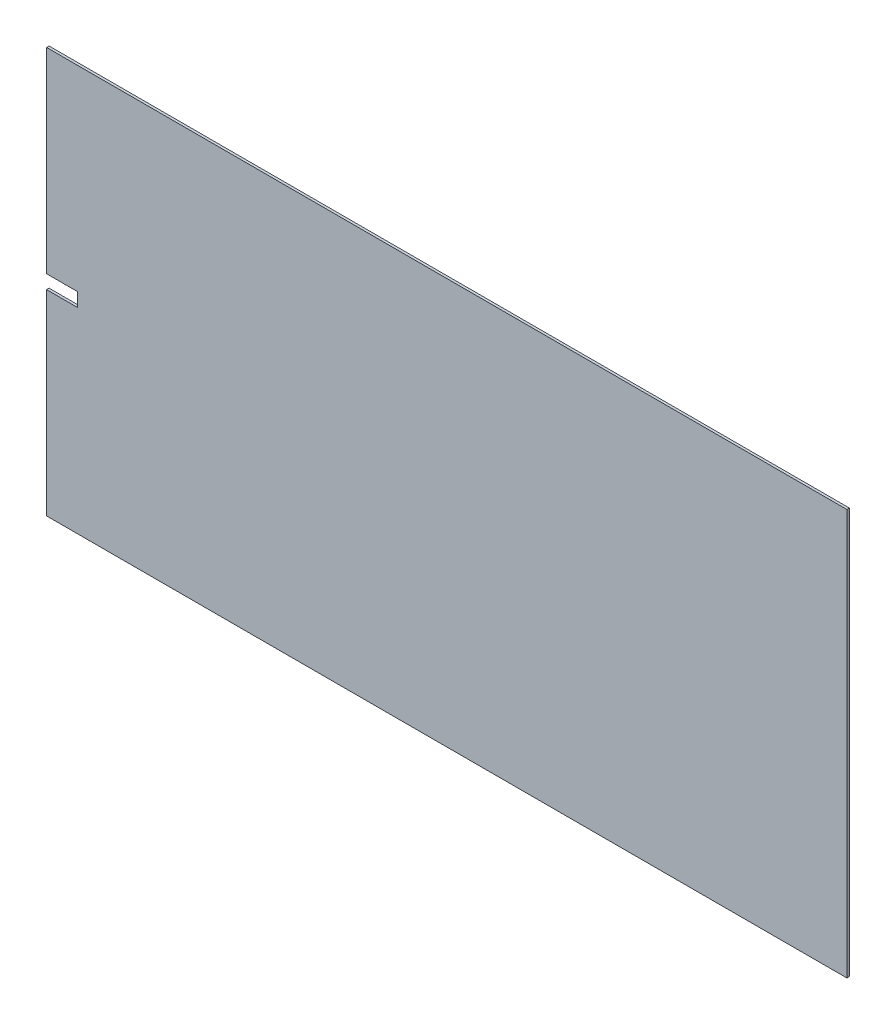
from build123d import *

# Parameters (mm, degrees)
BOSS_EXTRUDE1_DEPTH = 4


with BuildPart() as part:
    # Sketch1 → Boss-Extrude1 (new body)
    with BuildSketch(Plane.XY):
        Polygon((0, 315), (50, 315), (50, 337), (0, 337), (0, 652), (1286, 652), (1286, 0), (0, 0), align=None)
    extrude(amount=BOSS_EXTRUDE1_DEPTH)


solid = part.part
